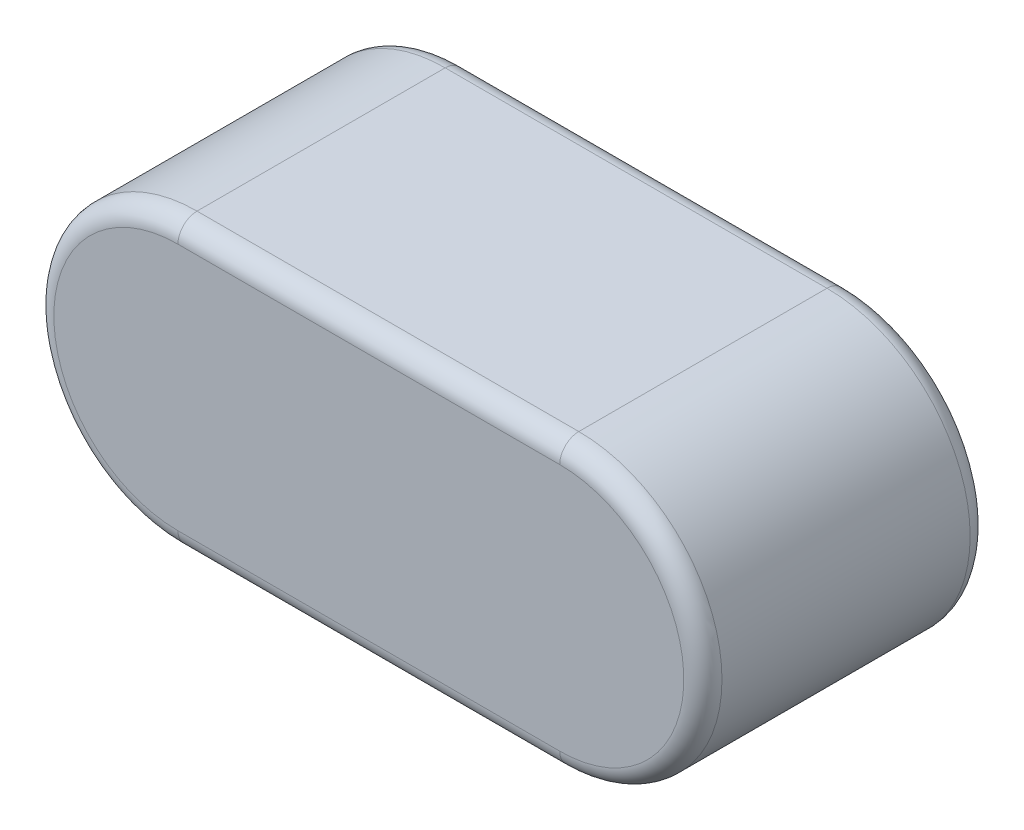
from build123d import *

# Parameters (mm, degrees)
EXTRUDE_523_DEPTH = 6
FILLET_1_R        = 0.4


with BuildPart() as part:
    # 草图1 → Extrude 523 (new body)
    with BuildSketch(Plane.XY):
        with BuildLine():
            Line((-4, 3), (4, 3))
            ThreePointArc((4, 3), (7, 0), (4, -3))
            Line((4, -3), (-4, -3))
            ThreePointArc((-4, -3), (-7, 0), (-4, 3))
        make_face()
    extrude(amount=EXTRUDE_523_DEPTH)

    # 圆角1
    fillet_1_edges = [part.edges().sort_by_distance(p)[0] for p in [
        (7, 0, 6),
        (0, 3, 6),
        (-7, 0, 6),
        (0, 3, 0),
        (7, 0, 0),
        (0, -3, 0),
        (-7, 0, 0),
        (0, -3, 6),
    ]]
    fillet(fillet_1_edges, radius=FILLET_1_R)


solid = part.part
